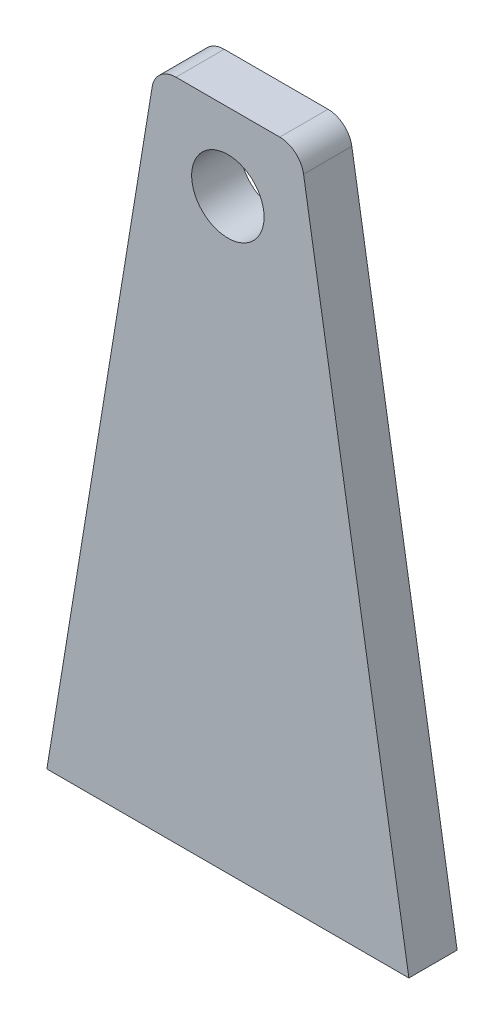
from build123d import *

# Parameters (mm, degrees)
SKETCH1_R           = 30
BOSS_EXTRUDE1_DEPTH = 40


with BuildPart() as part:
    # Sketch1 → Boss-Extrude1 (new body)
    with BuildSketch(Plane.XY):
        with BuildLine():
            Line((0, 0), (300, 0))
            Line((300, 0), (212.744219232, 533.229771362))
            ThreePointArc((212.744219232, 533.229771362), (205.956719326, 545.241316007), (193.006727574, 550))
            Line((193.006727574, 550), (106.993272426, 550))
            ThreePointArc((106.993272426, 550), (94.043280674, 545.241316007), (87.255780768, 533.229771362))
            Line((87.255780768, 533.229771362), (0, 0))
        make_face()
        with Locations((150, 486)):
            Circle(SKETCH1_R, mode=Mode.SUBTRACT)
    extrude(amount=BOSS_EXTRUDE1_DEPTH)


solid = part.part
